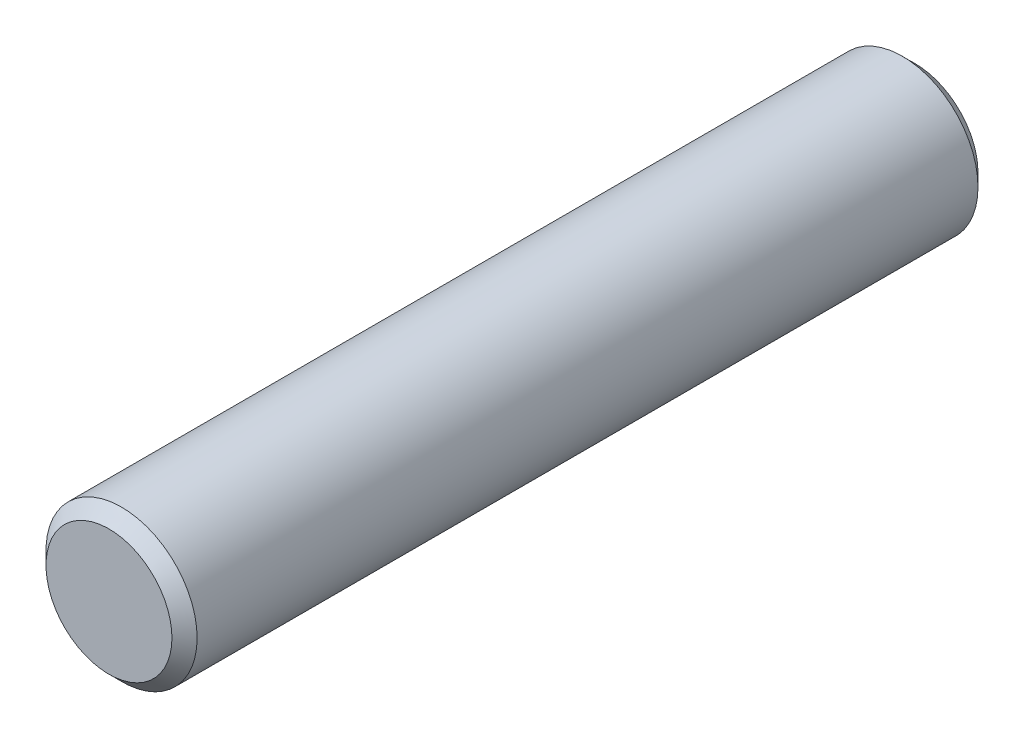
SolidWorks part; units mm, degrees
material "1023 碳钢板 (SS)"
ref_plane "前视基准面" through (0, 0, 0) normal (0, 0, 1) x (1, 0, 0)
ref_plane "上视基准面" through (0, 0, 0) normal (0, 1, 0) x (1, 0, 0)
ref_plane "右视基准面" through (0, 0, 0) normal (1, 0, 0) x (0, 0, -1)
sketch "草图1" plane through (0, 0, 0) normal (0, 0, 1) x (1, 0, 0)
  circle A0 centre (0, 0) radius 3
  dimension "D1" = 6
extrude "凸台-拉伸1" add sketch "草图1" along normal blind 32
chamfer "倒角1" distance 0.5 angle 45 2 edges at (3, 0, 32) (3, 0, 0)
ref_plane "基准面1" through (0, 0, 16) normal (0, 0, 1) x (1, 0, 0)
